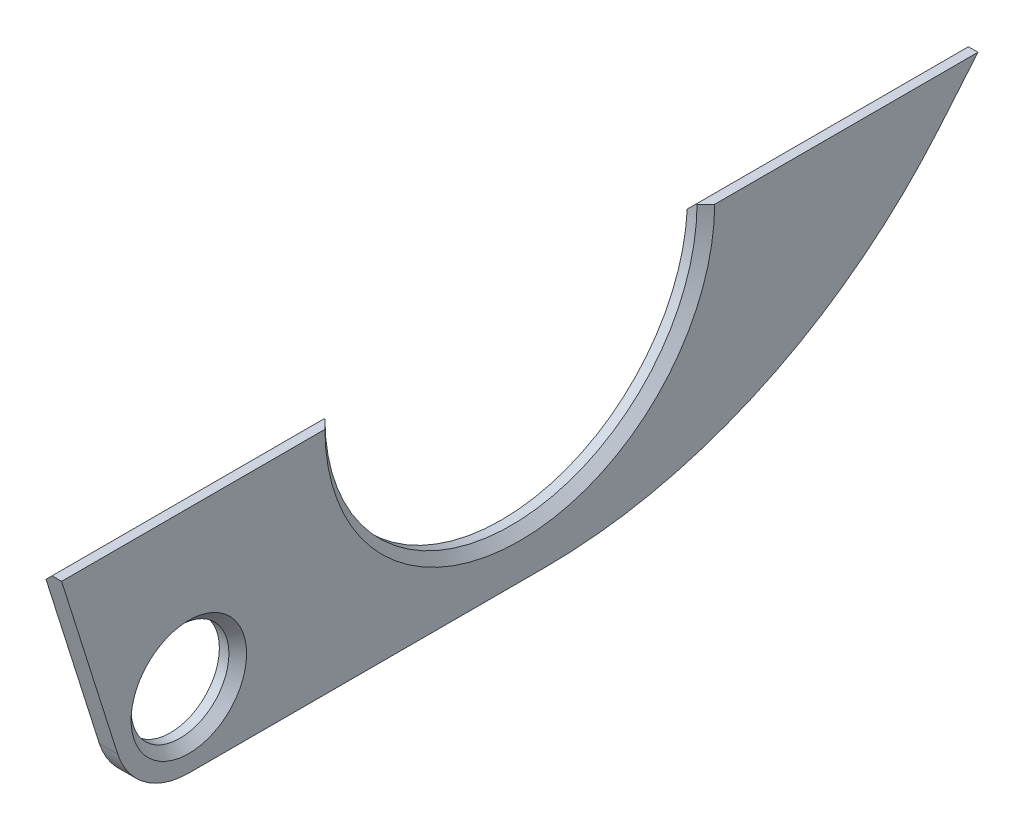
from build123d import *

# Parameters (mm, degrees)
BOSS_EXTRUDE1_DEPTH     = 12.5
CUT_EXTRUDE1_DEPTH      = 698.543905428
CUT_EXTRUDE1_DEPTH_BACK = 698.543905428
SKETCH2_R               = 66.5
FILLET1_R               = 700
CHAMFER1_SIZE           = 12
CHAMFER2_SIZE           = 12


with BuildPart() as part:
    # Sketch1 → Boss-Extrude1 (new, symmetric)
    with BuildSketch(Plane(origin=(0, 0, 0), x_dir=(0, 0, -1), z_dir=(1, 0, 0))):
        with BuildLine():
            Line((623, -1.2), (252.997154134, -1.2))
            ThreePointArc((252.997154134, -1.2), (0, -253), (-252.997154134, -1.2))
            Line((-252.997154134, -1.2), (-623, -1.2))
            Line((-623, -1.2), (-546.789689993, -242.561510288))
            ThreePointArc((-546.789689993, -242.561510288), (-510.001069598, -293.866486715), (-450, -313.5))
            Line((-450, -313.5), (360.949185183, -313.5))
            Line((360.949185183, -313.5), (623, -1.2))
        make_face()
    extrude(amount=BOSS_EXTRUDE1_DEPTH, both=True)

    # Sketch2 → Cut-Extrude1 (cut, two sides: drawn at the far end of the back side and taken through both)
    with BuildSketch(Plane(origin=(0, 0, 0), x_dir=(0, 0, -1), z_dir=(1, 0, 0)).offset(-CUT_EXTRUDE1_DEPTH_BACK)):
        with Locations((-450, -212)):
            Circle(SKETCH2_R)
    extrude(amount=CUT_EXTRUDE1_DEPTH + CUT_EXTRUDE1_DEPTH_BACK, mode=Mode.SUBTRACT)

    # Fillet1
    fillet1_edges = [part.edges().sort_by_distance(p)[0] for p in [
        (0, -313.5, -360.949185183),
    ]]
    fillet(fillet1_edges, radius=FILLET1_R)

    # Chamfer1
    chamfer1_edges = [part.edges().sort_by_distance(p)[0] for p in [
        (12.5, -212, 516.5),
        (12.5, -253, 0),
    ]]
    chamfer(chamfer1_edges, length=CHAMFER1_SIZE)

    # Chamfer2
    chamfer2_edges = [part.edges().sort_by_distance(p)[0] for p in [
        (-12.5, -1.2, -437.998577067),
        (-12.5, -1.2, 437.998577067),
    ]]
    chamfer(chamfer2_edges, length=CHAMFER2_SIZE)


solid = part.part
